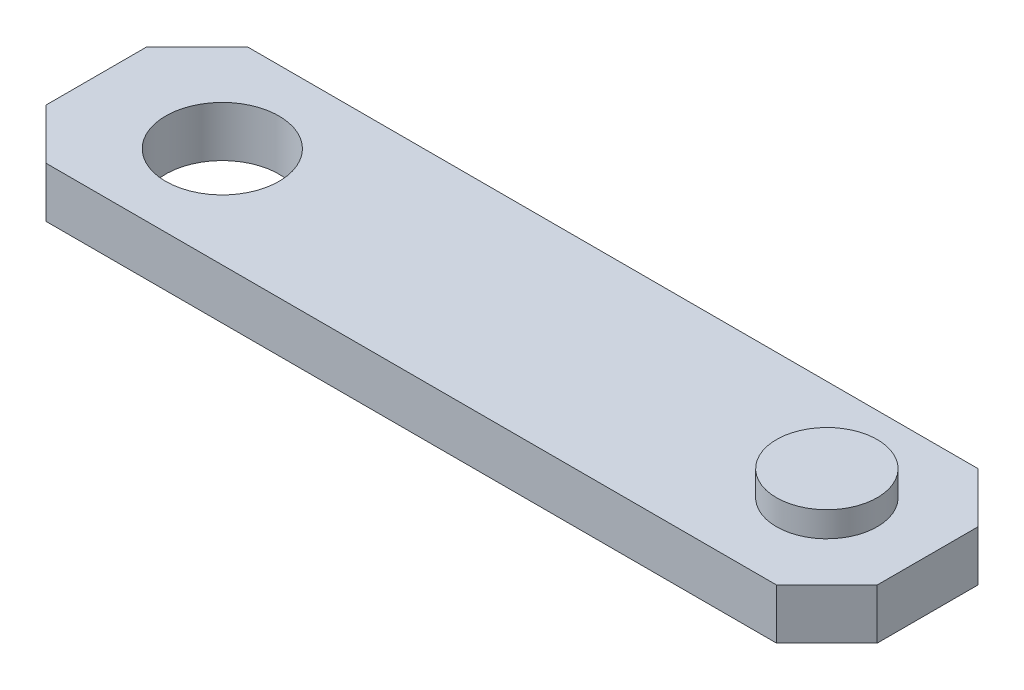
SolidWorks part; units mm, degrees
ref_plane "Front Plane" through (0, 0, 0) normal (0, 0, 1) x (1, 0, 0)
ref_plane "Top Plane" through (0, 0, 0) normal (0, 1, 0) x (1, 0, 0)
ref_plane "Right Plane" through (0, 0, 0) normal (1, 0, 0) x (0, 0, -1)
sketch "Sketch1" plane through (0, 0, 0) normal (0, 1, 0) x (1, 0, 0)
  line L1 (-9.6934, 7.4844) -> (23.3066, 7.4844)
  line L2 (-9.6934, 7.4844) -> (-9.6934, -0.5156)
  line L3 (-9.6934, -0.5156) -> (23.3066, -0.5156)
  line L4 (23.3066, 7.4844) -> (23.3066, -0.5156)
  dimension "D1" = 33
  dimension "D2" = 8
extrude "Boss-Extrude1" add sketch "Sketch1" along normal blind 2
sketch "Sketch2" plane through (0, 2, 0) normal (0, 1, 0) x (1, 0, 0)
  line L0 (23.3066, 7.4844) -> (-9.6934, 7.4844) construction
  line L1 (-9.6934, 7.4844) -> (-9.6934, -0.5156) construction
  circle A0 centre (-4.6934, 3.4844) radius 2.25
  dimension "D3" = 4.5
  dimension "D1" = 4
  dimension "D2" = 5
extrude "Cut-Extrude1" cut sketch "Sketch2" against normal through all
sketch "Sketch3" plane through (0, 2, 0) normal (0, 1, 0) x (1, 0, 0)
  line L0 (23.3066, 7.4844) -> (-9.6934, 7.4844) construction
  line L1 (23.3066, -0.5156) -> (23.3066, 7.4844) construction
  circle A0 centre (19.3066, 3.4844) radius 2
  dimension "D2" = 4
  dimension "D3" = 4
  dimension "D1" = 4
extrude "Boss-Extrude2" add sketch "Sketch3" along normal blind 1
chamfer "Chamfer1" [suppressed] distance 0.5 angle 45
chamfer "Chamfer2" distance 2 angle 45 4 edges at (23.3066, 1, -7.4844) (23.3066, 1, 0.5156) (-9.6934, 1, 0.5156) (-9.6934, 1, -7.4844)
